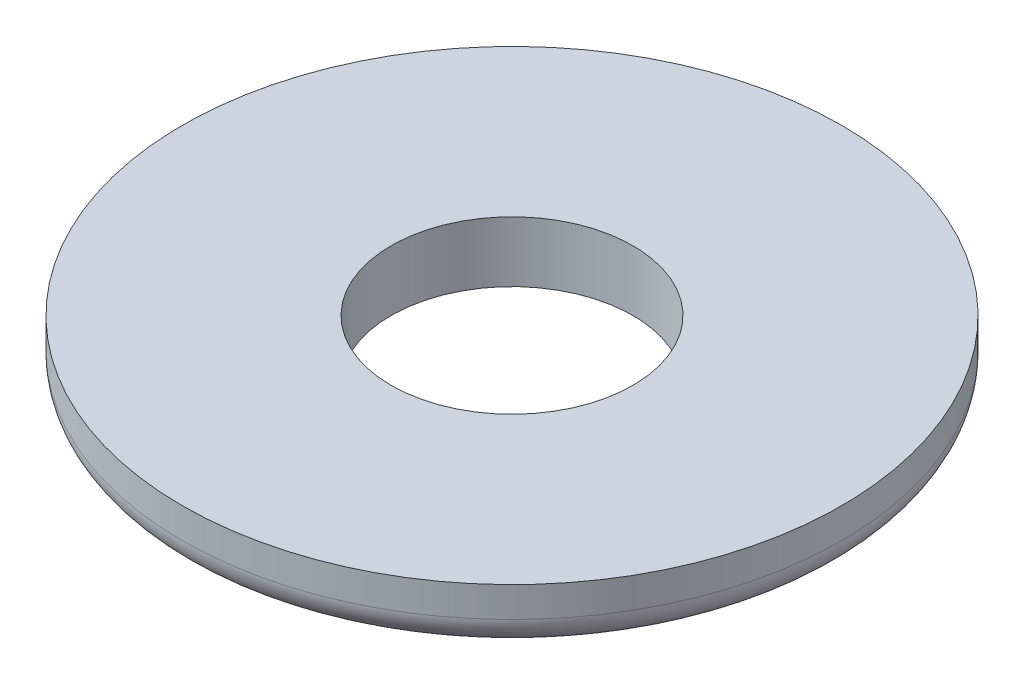
from build123d import *


with BuildPart() as part:
    # 草图1 → 旋转1 (revolve)
    with BuildSketch(Plane.XY, mode=Mode.PRIVATE) as revolve_1_sk:
        with BuildLine():
            Line((20, -7.047028188), (49.5, -7.047028188))
            ThreePointArc((49.5, -7.047028188), (53.035533906, -5.582562094), (54.5, -2.047028188))
            Line((54.5, -2.047028188), (54.5, 2.952971812))
            Line((54.5, 2.952971812), (20, 2.952971812))
            Line((20, 2.952971812), (20, -7.047028188))
        make_face()
    revolve(revolve_1_sk.sketch.rotate(Axis((0, 51.82089634, 0), (0, -1, 0)), 90), axis=Axis((0, 51.82089634, 0), (0, -1, 0)))


solid = part.part
